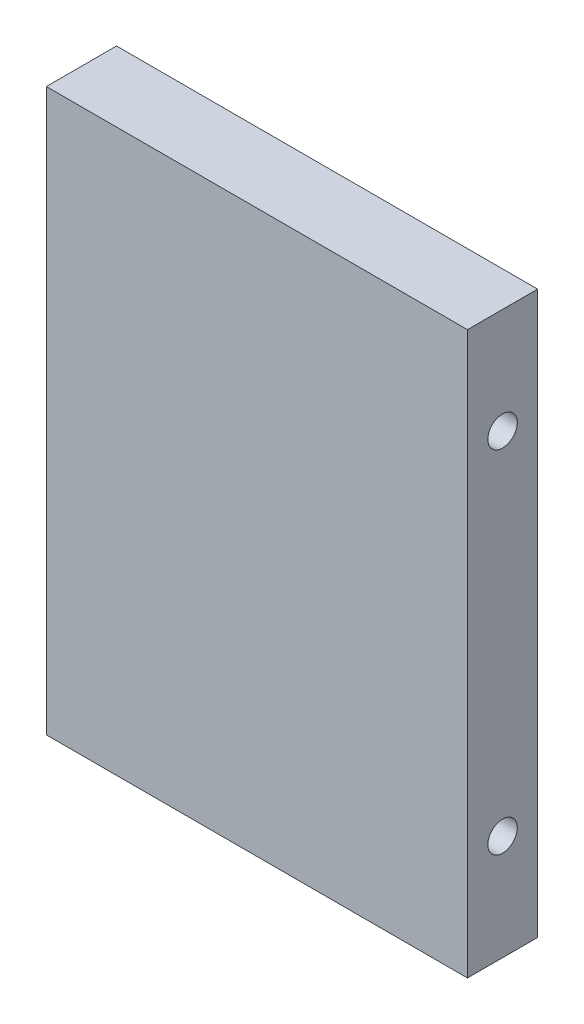
from build123d import *

# Parameters (mm, degrees)
SKETCH_1_W             = 60
SKETCH_1_H             = 80
EXTRUDE_1_DEPTH        = 10
HOLE_WIZARD_M5_1_D     = 4.2
HOLE_WIZARD_M5_1_DEPTH = 14
HOLE_WIZARD_M5_1_TIP   = 1.2618073
HOLE_WIZARD_M5_2_D     = 4.2
HOLE_WIZARD_M5_2_DEPTH = 14
HOLE_WIZARD_M5_2_TIP   = 1.2618073


with BuildPart() as part:
    # 草图1 → 凸台-拉伸1 (new body)
    with BuildSketch(Plane.XY):
        Rectangle(SKETCH_1_W, SKETCH_1_H)
    extrude(amount=EXTRUDE_1_DEPTH)

    # M5 螺纹孔1
    with Locations(Plane(origin=(30, 0, 0), x_dir=(0, 0, -1), z_dir=(1, 0, 0))):
        with Locations((-5, -25), (-5, 25)):
            Hole(HOLE_WIZARD_M5_1_D / 2, depth=HOLE_WIZARD_M5_1_DEPTH)
            with Locations((0, 0, -(HOLE_WIZARD_M5_1_DEPTH + HOLE_WIZARD_M5_1_TIP / 2))):  # 118° drill point
                Cone(0, HOLE_WIZARD_M5_1_D / 2, HOLE_WIZARD_M5_1_TIP, mode=Mode.SUBTRACT)

    # M5 螺纹孔2
    with Locations(Plane.ZY.offset(30)):
        with Locations((5, 25), (5, -25)):
            Hole(HOLE_WIZARD_M5_2_D / 2, depth=HOLE_WIZARD_M5_2_DEPTH)
            with Locations((0, 0, -(HOLE_WIZARD_M5_2_DEPTH + HOLE_WIZARD_M5_2_TIP / 2))):  # 118° drill point
                Cone(0, HOLE_WIZARD_M5_2_D / 2, HOLE_WIZARD_M5_2_TIP, mode=Mode.SUBTRACT)


solid = part.part
